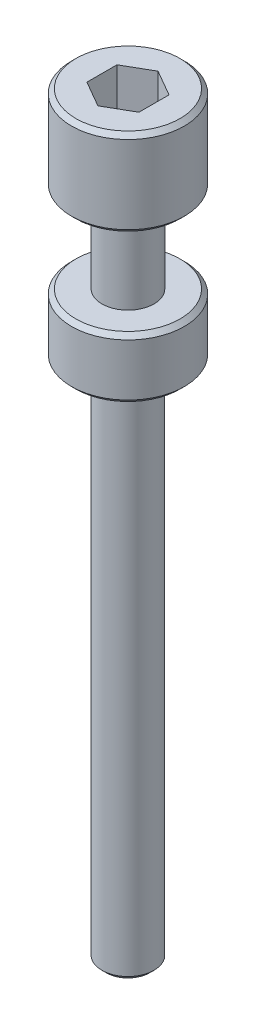
from build123d import *

# Parameters (mm, degrees)
SKETCH1_R           = 3
BOSS_EXTRUDE1_DEPTH = 45
SKETCH2_R           = 3
BOSS_EXTRUDE2_DEPTH = 15
SKETCH3_R           = 6.5
BOSS_EXTRUDE3_DEPTH = 7
SKETCH4_R           = 3
BOSS_EXTRUDE4_DEPTH = 10
SKETCH5_R           = 6.5
BOSS_EXTRUDE5_DEPTH = 10
CUT_EXTRUDE1_DEPTH  = 6
CHAMFER1_SIZE       = 0.5


with BuildPart() as part:
    # Sketch1 → Boss-Extrude1 (new body)
    with BuildSketch(Plane(origin=(0, 0, 0), x_dir=(1, 0, 0), z_dir=(0, 1, 0))):
        with Locations(Location((0, 0, 0), (0, 0, 90))):
            Circle(SKETCH1_R)
    extrude(amount=BOSS_EXTRUDE1_DEPTH)

    # Sketch2 → Boss-Extrude2 (add)
    with BuildSketch(Plane(origin=(0, 45, 0), x_dir=(1, 0, 0), z_dir=(0, 1, 0))):
        with Locations(Location((0, 0, 0), (0, 0, 90))):
            Circle(SKETCH2_R)
    extrude(amount=BOSS_EXTRUDE2_DEPTH)

    # Sketch3 → Boss-Extrude3 (add)
    with BuildSketch(Plane(origin=(0, 60, 0), x_dir=(1, 0, 0), z_dir=(0, 1, 0))):
        with Locations(Location((0, 0, 0), (0, 0, 270))):
            Circle(SKETCH3_R)
    extrude(amount=BOSS_EXTRUDE3_DEPTH)

    # Sketch4 → Boss-Extrude4 (add)
    with BuildSketch(Plane(origin=(0, 67, 0), x_dir=(1, 0, 0), z_dir=(0, 1, 0))):
        with Locations(Location((0, 0, 0), (0, 0, 90))):
            Circle(SKETCH4_R)
    extrude(amount=BOSS_EXTRUDE4_DEPTH)

    # Sketch5 → Boss-Extrude5 (add)
    with BuildSketch(Plane(origin=(0, 77, 0), x_dir=(1, 0, 0), z_dir=(0, 1, 0))):
        with Locations(Location((0, 0, 0), (0, 0, 270))):
            Circle(SKETCH5_R)
    extrude(amount=BOSS_EXTRUDE5_DEPTH)

    # Sketch6 → Cut-Extrude1 (cut)
    with BuildSketch(Plane(origin=(0, 87, 0), x_dir=(1, 0, 0), z_dir=(0, 1, 0))):
        Polygon((0, 3.464101615), (-3, 1.732050808), (-3, -1.732050808), (0, -3.464101615), (3, -1.732050808), (3, 1.732050808), align=None)
    extrude(amount=-CUT_EXTRUDE1_DEPTH, mode=Mode.SUBTRACT)

    # Chamfer1
    chamfer1_edges = [part.edges().sort_by_distance(p)[0] for p in [
        (0, 77, -6.5),
        (0, 87, -6.5),
        (0, 0, 3),
        (0, 60, -6.5),
        (0, 67, -6.5),
    ]]
    chamfer(chamfer1_edges, length=CHAMFER1_SIZE)


solid = part.part
